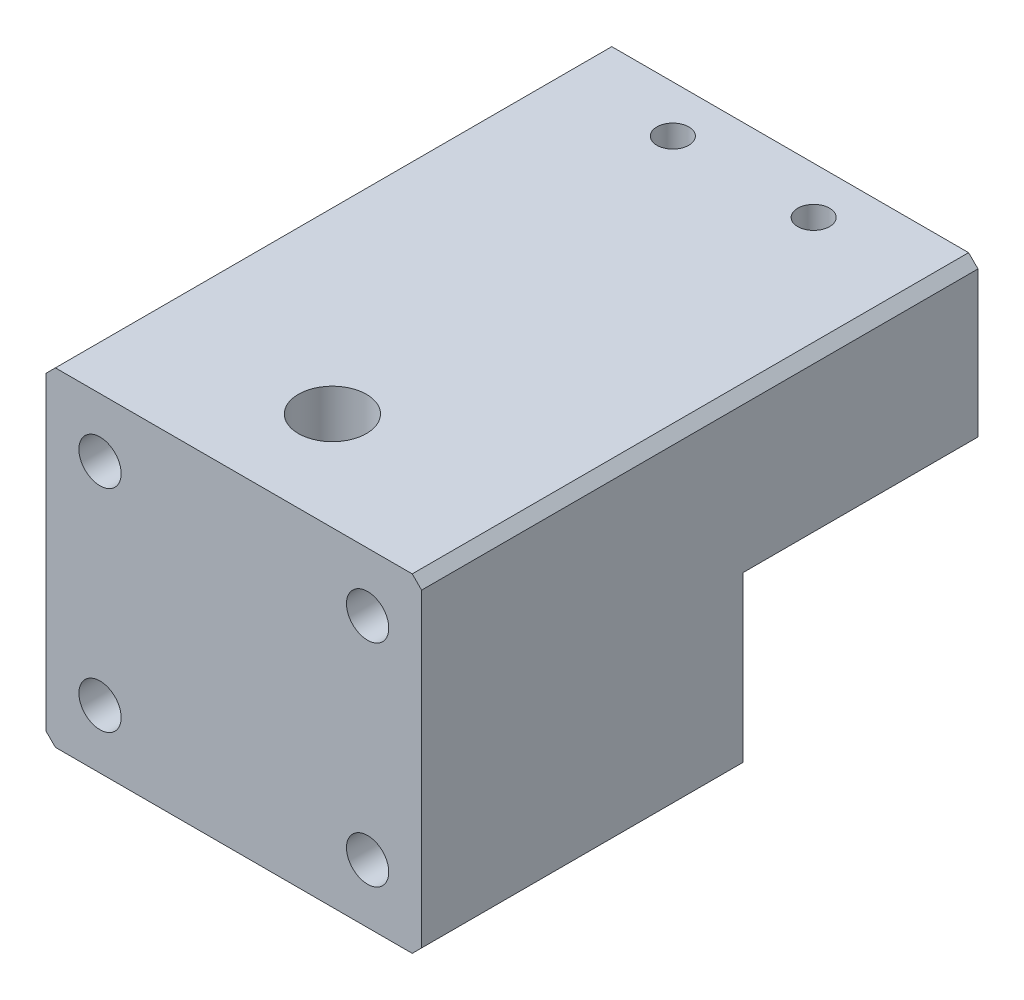
from build123d import *

# Parameters (mm, degrees)
SKETCH_1_W             = 80
SKETCH_1_H             = 70
EXTRUDE_1_DEPTH        = 118.5
SKETCH_4_R             = 7
CUT_EXTRUDE_1_DEPTH    = 80
SKETCH_5_R             = 4.5
CUT_EXTRUDE_2_DEPTH    = 160.192493542
SKETCH_6_W             = 80
SKETCH_6_H             = 35
CUT_EXTRUDE_3_DEPTH    = 50
M16X1_5_1_D            = 14.5
M16X1_5_1_DEPTH        = 36.5
M16X1_5_1_TIP          = 4.356239488
HOLE_WIZARD_M8_1_D     = 6.8
HOLE_WIZARD_M8_1_DEPTH = 19.75
HOLE_WIZARD_M8_1_TIP   = 2.042926105
CHAMFER_1_SIZE         = 2


with BuildPart() as part:
    # 草图1 → 凸台-拉伸1 (new body)
    with BuildSketch(Plane.XY):
        with Locations((40, 35)):
            Rectangle(SKETCH_1_W, SKETCH_1_H)
    extrude(amount=EXTRUDE_1_DEPTH)

    # 草图4 → 切除-拉伸1 (cut)
    with BuildSketch(Plane(origin=(0, 0, 0), x_dir=(-1, 0, 0), z_dir=(0, 0, -1))):
        with Locations((-11.5, 57.5)):
            Circle(SKETCH_4_R)
        with Locations((-11.5, 12.5)):
            Circle(SKETCH_4_R)
        with Locations((-68.5, 57.5)):
            Circle(SKETCH_4_R)
        with Locations((-68.5, 12.5)):
            Circle(SKETCH_4_R)
    extrude(amount=-CUT_EXTRUDE_1_DEPTH, mode=Mode.SUBTRACT)

    # 草图5 → 切除-拉伸2 (cut, through all)
    with BuildSketch(Plane(origin=(0, 0, 0), x_dir=(-1, 0, 0), z_dir=(0, 0, -1))):
        with Locations((-68.5, 57.5)):
            Circle(SKETCH_5_R)
        with Locations((-11.5, 57.5)):
            Circle(SKETCH_5_R)
        with Locations((-11.5, 12.5)):
            Circle(SKETCH_5_R)
        with Locations((-68.5, 12.5)):
            Circle(SKETCH_5_R)
    extrude(amount=-CUT_EXTRUDE_2_DEPTH, mode=Mode.SUBTRACT)

    # 草图6 → 切除-拉伸3 (cut)
    with BuildSketch(Plane(origin=(0, 0, 0), x_dir=(-1, 0, 0), z_dir=(0, 0, -1))):
        with Locations((-40, 17.5)):
            Rectangle(SKETCH_6_W, SKETCH_6_H)
    extrude(amount=-CUT_EXTRUDE_3_DEPTH, mode=Mode.SUBTRACT)

    # M16x1.5 螺纹孔1
    with Locations(Plane(origin=(0, 70, 0), x_dir=(1, 0, 0), z_dir=(0, 1, 0))):
        with Locations((40, -97.5)):
            Hole(M16X1_5_1_D / 2, depth=M16X1_5_1_DEPTH)
            with Locations((0, 0, -(M16X1_5_1_DEPTH + M16X1_5_1_TIP / 2))):  # 118° drill point
                Cone(0, M16X1_5_1_D / 2, M16X1_5_1_TIP, mode=Mode.SUBTRACT)

    # M8 螺纹孔1
    with Locations(Plane(origin=(0, 70, 0), x_dir=(1, 0, 0), z_dir=(0, 1, 0))):
        with Locations((55, -10), (25, -10)):
            Hole(HOLE_WIZARD_M8_1_D / 2, depth=HOLE_WIZARD_M8_1_DEPTH)
            with Locations((0, 0, -(HOLE_WIZARD_M8_1_DEPTH + HOLE_WIZARD_M8_1_TIP / 2))):  # 118° drill point
                Cone(0, HOLE_WIZARD_M8_1_D / 2, HOLE_WIZARD_M8_1_TIP, mode=Mode.SUBTRACT)

    # 倒角1
    chamfer_1_edges = [part.edges().sort_by_distance(p)[0] for p in [
        (80, 35, 25),
        (0, 35, 25),
        (0, 70, 59.25),
        (80, 70, 59.25),
        (80, 0, 84.25),
        (0, 0, 84.25),
    ]]
    chamfer(chamfer_1_edges, length=CHAMFER_1_SIZE)


solid = part.part
